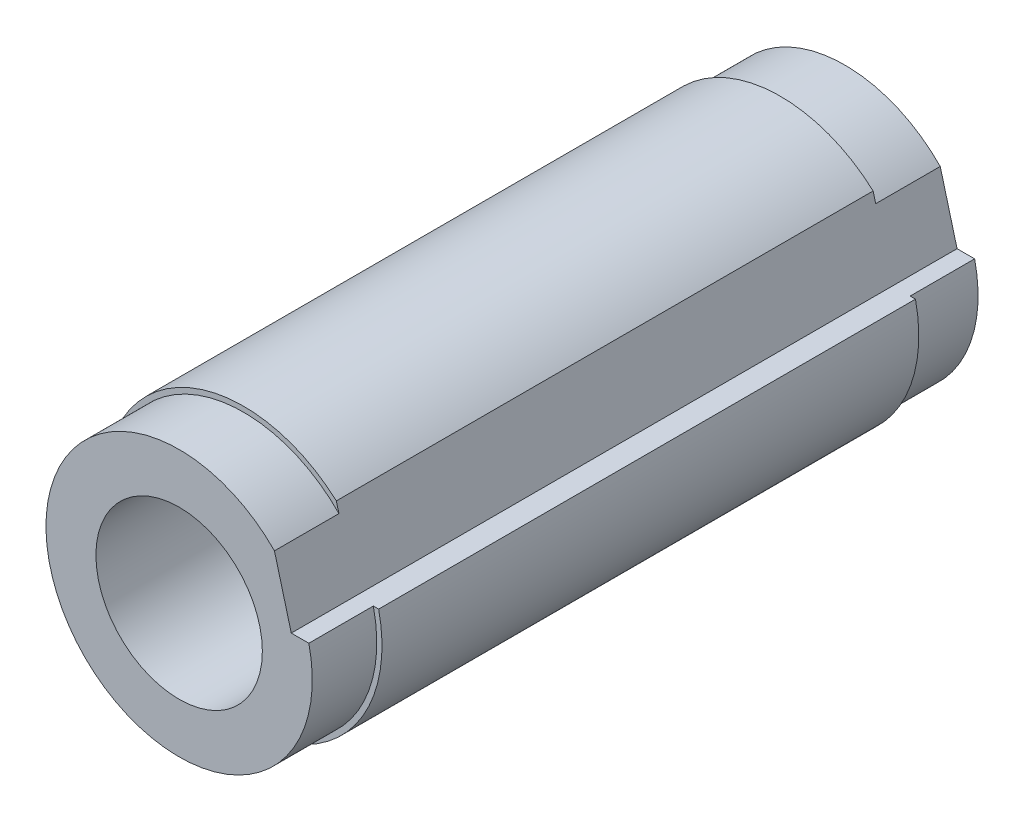
from build123d import *

# Parameters (mm, degrees)
SKETCH1_R           = 66.5
SKETCH1_R_2         = 36.5
BOSS_EXTRUDE1_DEPTH = 320
SKETCH3_R           = 40
CUT_EXTRUDE1_DEPTH  = 79.7
CUT_EXTRUDE2_START  = -31
SKETCH4_R           = 66.5
SKETCH4_R_2         = 64
CUT_EXTRUDE2_DEPTH  = 31
CUT_EXTRUDE3_DEPTH  = 334.533356653


with BuildPart() as part:
    # Sketch1 → Boss-Extrude1 (new body)
    with BuildSketch(Plane.XY):
        Circle(SKETCH1_R)
        Circle(SKETCH1_R_2, mode=Mode.SUBTRACT)
    extrude(amount=BOSS_EXTRUDE1_DEPTH)

    # Sketch3 → Cut-Extrude1 (cut)
    with BuildSketch(Plane.XY.offset(320)):
        Circle(SKETCH3_R)
    cut_extrude1 = extrude(amount=-CUT_EXTRUDE1_DEPTH, mode=Mode.SUBTRACT)

    # Sketch4 → Cut-Extrude2 (cut)
    with BuildSketch(Plane.XY.offset(320).offset(CUT_EXTRUDE2_START)):
        Circle(SKETCH4_R)
        Circle(SKETCH4_R_2, mode=Mode.SUBTRACT)
    cut_extrude2 = extrude(amount=CUT_EXTRUDE2_DEPTH, mode=Mode.SUBTRACT)

    # Mirror1: Cut-Extrude1, Cut-Extrude2 across plane
    add(cut_extrude1.mirror(Plane.XY.offset(160)), mode=Mode.SUBTRACT)
    add(cut_extrude2.mirror(Plane.XY.offset(160)), mode=Mode.SUBTRACT)

    # Sketch5 → Cut-Extrude3 (cut, through all)
    with BuildSketch(Plane.XY.offset(320)):
        with BuildLine():
            Line((64.899922958, 14.5), (53.899922958, 14.5))
            Line((53.899922958, 14.5), (44.558079818, 49.364233235))
            ThreePointArc((44.558079818, 49.364233235), (57.43816051, 33.512799305), (64.899922958, 14.5))
        make_face()
    extrude(amount=-CUT_EXTRUDE3_DEPTH, mode=Mode.SUBTRACT)


solid = part.part
